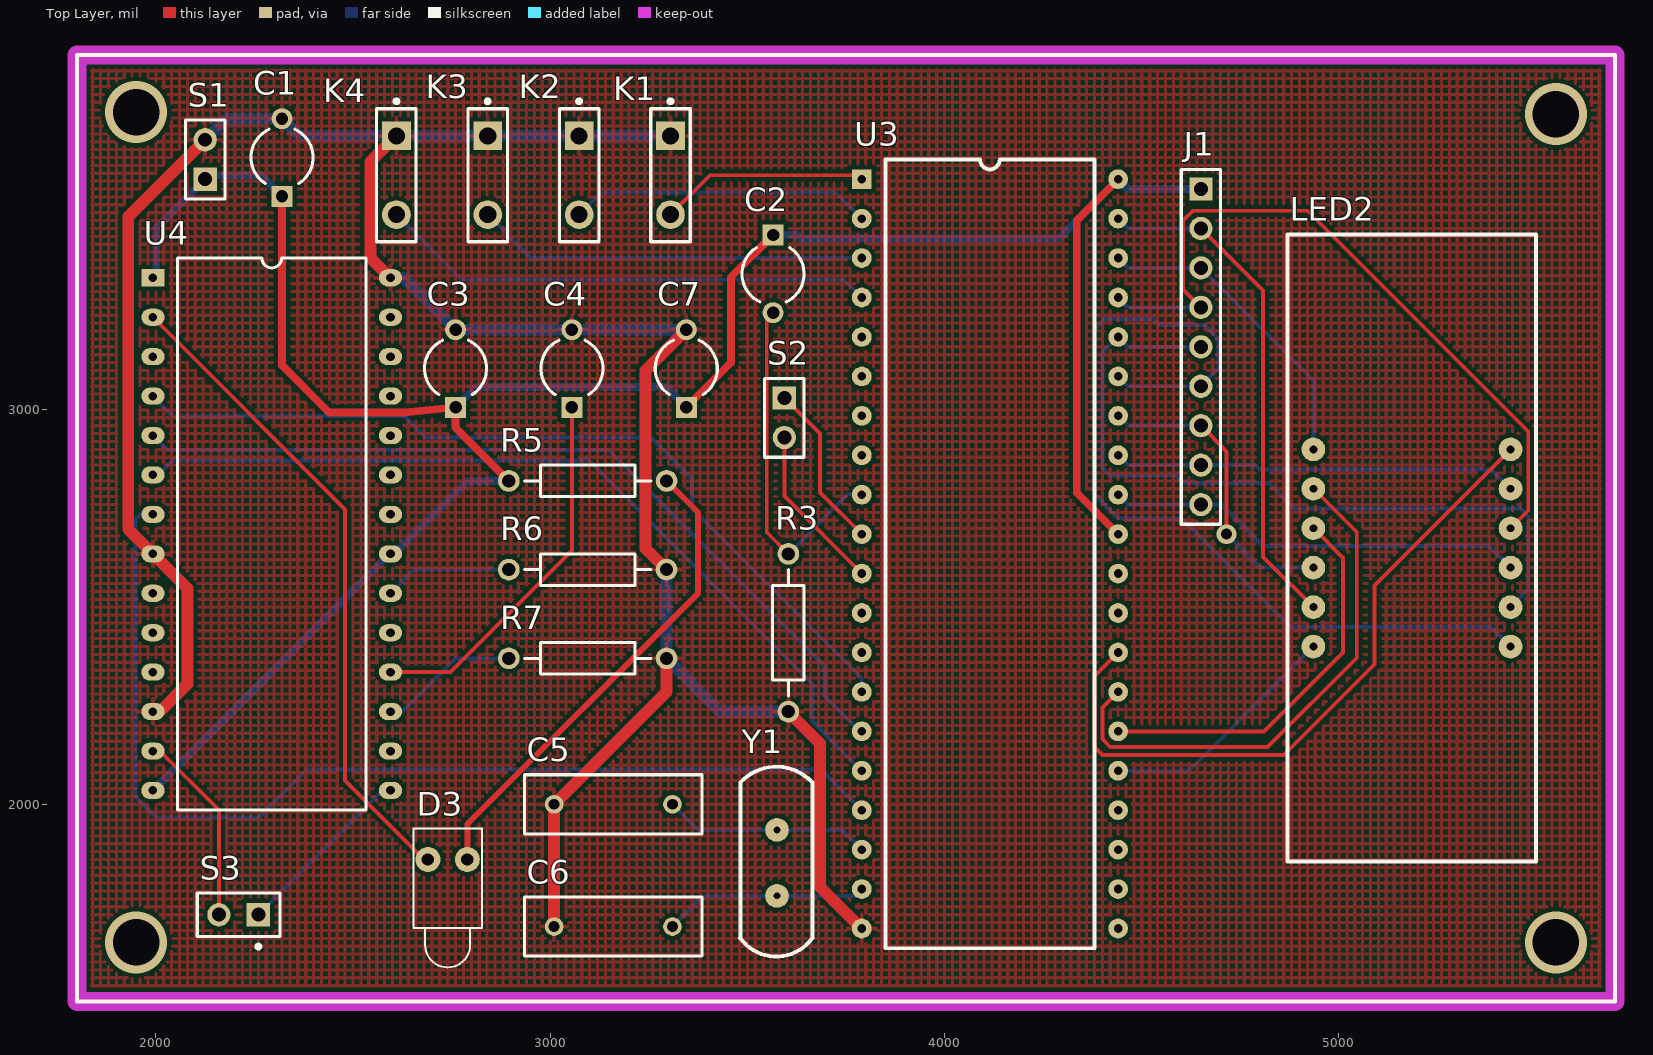
[diagram p0: Top Layer view]
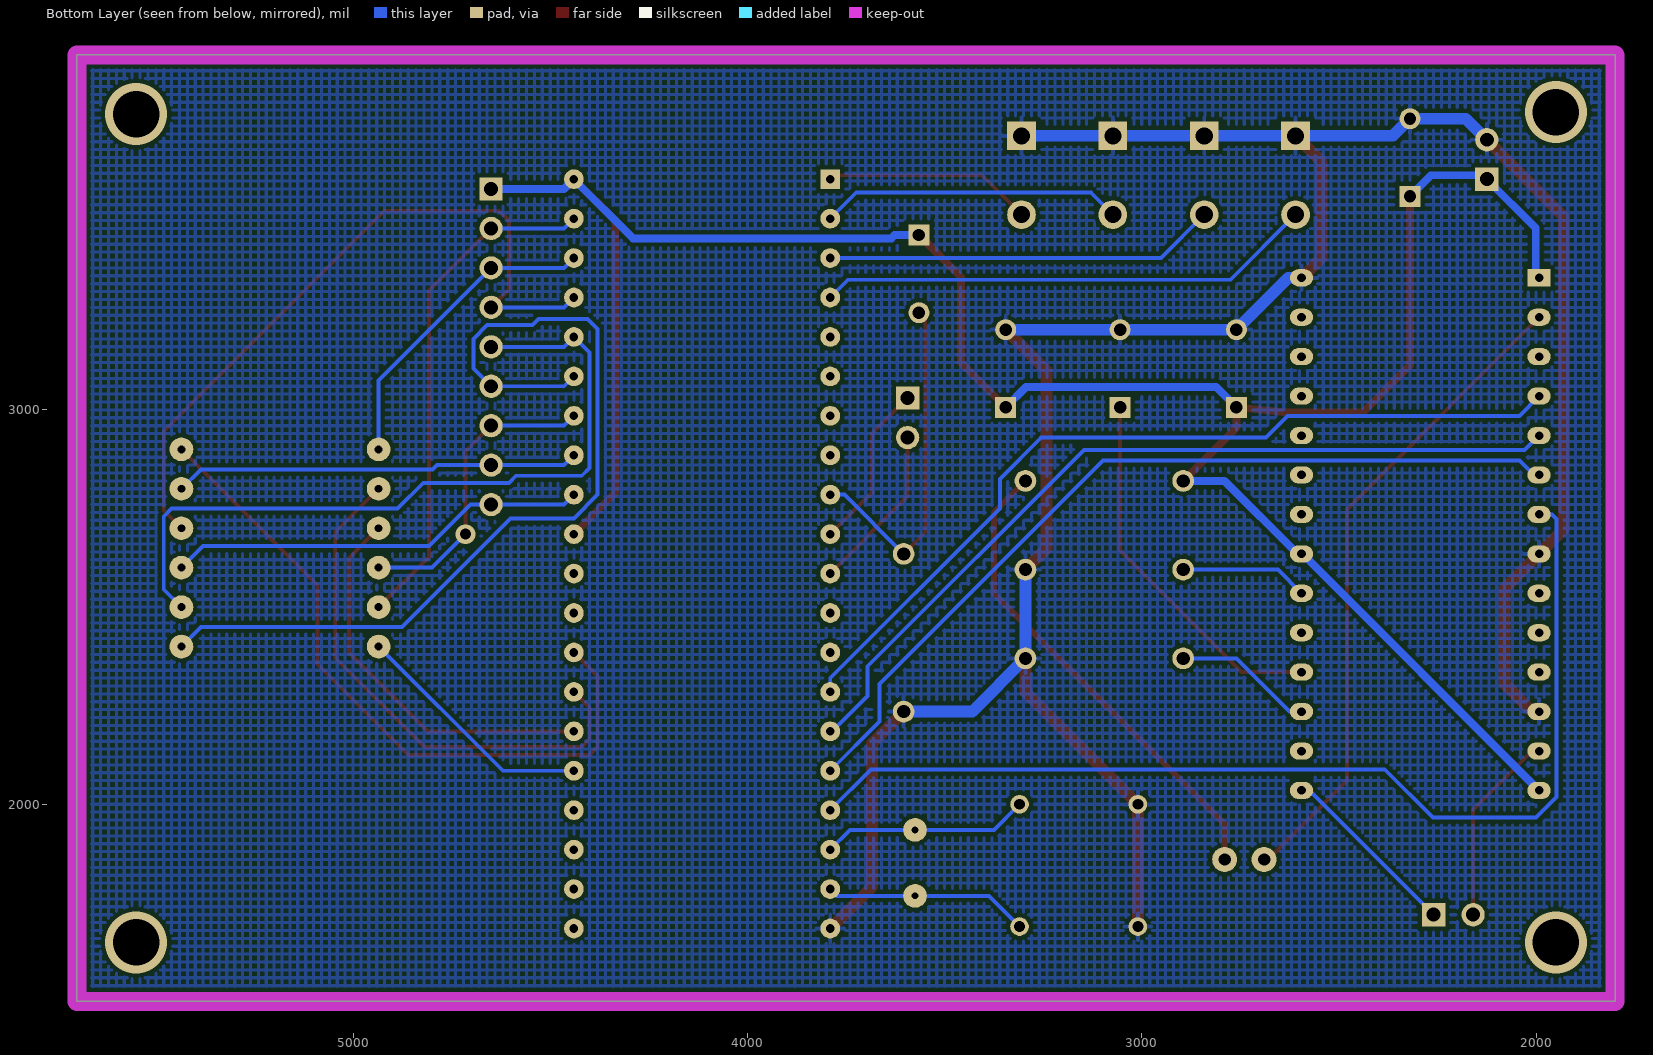
[diagram p1: Bottom Layer view, seen from below]
# Altium PCB MISC86338.PcbDoc
Units mil, origin at the board's own origin, x right, y up, seen from the top; angles counter-clockwise.
Board outline 3900 x 2400 mil, 2 copper layers (Top Layer, Bottom Layer); 24 components, 34 nets, 129 pads, 5 vias.

## Layer stack, top to bottom (the 12.6 mil dielectric is the usual default, probably not edited)
Top Solder: solder mask 0.4, Solder Resist, Dk 3.5
Top Layer: signal copper 1.4
Dielectric 1: dielectric 12.6, FR-4, Dk 4.8
Bottom Layer: signal copper 1.4
Bottom Solder: solder mask 0.4, Solder Resist, Dk 3.5

## Board outline
1800,1500 5700,1500 5700,3900 1800,3900

## Design rules (kind name [scope] priority, off if disabled: settings)
Clearance [All] p1: gap=10
HoleSize [All] p1: absolutevalues=TRUE maxlimit=500 minlimit=1 maxpercent=80.000 minpercent=20.000
MinimumSolderMaskSliver [All] p1: minsoldermaskwidth=5
PolygonConnect [All] p1: connectstyle=Relief reliefconductorwidth=10 reliefentries=4 polygonreliefangle="90 Angle" airgapwidth=10
RoomDefinition 公交自动报站器 [InComponentClass('公交自动报站器')] p1: confinementstyle=ConfineIn formatcopy=TRUE lockcomponents=FALSE outline 1800,1500 5700,1500 5700,3900 1800,3900
RoutingVias [All] p1: holewidth=28 width=50 viastyle="Through Hole" minholewidth=28 minwidth=50 maxholewidth=28 maxwidth=50
SilkToSolderMaskClearance [IsPad] p1: minsilkscreentomaskgap=0 clearancetoexposedcopper=TRUE
SolderMaskExpansion [All] p1: expansion=4
Width GND [InNet('GND')] p1: maxlimit=35 minlimit=10 preferedwidth=30
Width VCC [InNet('VCC')] p2: maxlimit=25 minlimit=10 preferedwidth=20
Width [All] p3: maxlimit=15 minlimit=8 preferedwidth=10
27 further rules are at their usual default settings.

## Components (designator, comment, footprint, x,y, rotation, side; value= is the part's Value field where it differs from the comment)
C1 "Cap2" CAPR5-4X5 2320,3640 r90 top
C2 "Cap2" CAPR5-4X5 3565,3345 r270 top
C3 "Cap2" CAPR5-4X5 2760,3105 r90 top
C4 "Cap2" CAPR5-4X5 3055,3105 r90 top
C5 "Cap" RAD-0.3 3160,2000 r0 top
C6 "Cap" RAD-0.3 3160,1690 r0 top
C7 "Cap2" CAPR5-4X5 3345,3105 r90 top
D3 "LED1" LED-1 2740,1860 r270 top
J1 "Header 9" HDR1X9 4650,3560 r270 top
K1 "SW-PB" SPST-2 3305,3595 r270 top
K2 "SW-PB" SPST-2 3073.33,3595 r270 top
K3 "SW-PB" SPST-2 2841.67,3595 r270 top
K4 "SW-PB" SPST-2 2610,3595 r270 top
LED2 "Dpy Red-CA" 四位数码管 5499.96,1854.72 r90 top
R3 "Res2" AXIAL-0.4 3603.74,2435 r90 top
R5 "Res2" AXIAL-0.4 3095,2820 r0 top
R6 "Res2" AXIAL-0.4 3095,2595 r180 top
R7 "Res2" AXIAL-0.4 3095,2370 r180 top
S1 "Header 2" HDR1X2 2125,3585 r90 top
S2 "Header 2" HDR1X2 3593.74,3030 r270 top
S3 "Speaker" PIN2 2260,1720 r180 top
U3 "89c51" 89c51 3790,3585 r0 top
U4 "Component_1" ISD1730 1992.64,3335 r0 top
Y1 "Component_1" XTAL 3665,2055 r180 top

## Footprints (in the part's own frame and the unit in brackets; to place one, negate y for a bottom-side part, rotate by r counter-clockwise, add the part's x,y. Pads: shape width x height; smd on the part's side, far side on the other; paste and mask are expansions set on the pad)
89c51 [mil]
  rect 50x50 hole 22: 1(0,0)
  round 50 hole 22: 2(0,-100) 3(0,-200) 4(0,-300) 5(0,-400) 6(0,-500) 7(0,-600) 8(0,-700) 9(0,-800) 10(0,-900) 11(0,-1000) 12(0,-1100) 13(0,-1200) 14(0,-1300) 15(0,-1400) 16(0,-1500) 17(0,-1600) 18(0,-1700) 19(0,-1800) 20(0,-1900) 21(650,-1900) 22(650,-1800) 23(650,-1700) 24(650,-1600) 25(650,-1500) 26(650,-1400) 27(650,-1300) 28(650,-1200) 29(650,-1100) 30(650,-1000) 31(650,-900) 32(650,-800) 33(650,-700) 34(650,-600) 35(650,-500) 36(650,-400) 37(650,-300) 38(650,-200) 39(650,-100) 40(650,0)
  silkscreen extent 60,-1950 590,50, body extent 65,-1950 590,55, height 190
AXIAL-0.4 [mm] "Axial Device, Thru-Hole; 2 Leads; 0.4 in Pin Spacing"
  round 1.4 hole 0.85: 1(-5.08,0) 2(5.08,0)
  silkscreen extent -4.06,-1.02 4.06,1.02
CAPR5-4X5 [mm] "Capacitor; 2 Leads"
  rect 1.35x1.35 hole 0.8: 1(-2.5,0)
  round 1.35 hole 0.8: 2(2.5,0)
  silkscreen extent -1.69,-2 1.82,2
HDR1X2 [mm] "Connector; Header; 2 Position"
  rect 1.5x1.5 hole 0.9: 1(0,0)
  round 1.5 hole 0.9: 2(2.54,0)
  silkscreen extent -1.27,-1.27 3.81,1.27
HDR1X9 [mm] "Connector; Header; 9 Position"
  rect 1.5x1.5 hole 0.9: 1(0,0)
  round 1.5 hole 0.9: 2(2.54,0) 3(5.08,0) 4(7.62,0) 5(10.16,0) 6(12.7,0) 7(15.24,0) 8(17.78,0) 9(20.32,0)
  silkscreen extent -1.27,-1.27 21.59,1.27
ISD1730 [mm]
  rect 1.5x1.1 hole 0.55: 1(0,0)
  oval 1.5x1.1 hole 0.55: 2(0,-2.54) 3(0,-5.08) 4(0,-7.62) 5(0,-10.16) 6(0,-12.7) 7(0,-15.24) 8(0,-17.78) 9(0,-20.32) 10(0,-22.86) 11(0,-25.4) 12(0,-27.94) 13(0,-30.48) 14(0,-33.02) 15(15.3,-33.02) 16(15.3,-30.48) 17(15.3,-27.94) 18(15.3,-25.4) 19(15.3,-22.86) 20(15.3,-20.32) 21(15.3,-17.78) 22(15.3,-15.24) 23(15.3,-12.7) 24(15.3,-10.16) 25(15.3,-7.62) 26(15.3,-5.08) 27(15.3,-2.54) 28(15.3,0)
  silkscreen extent 1.59,-34.29 13.71,1.27
LED-1 [mm] "LED; 2 Leads"
  round 1.6 hole 0.8: 1(0,1.27) 2(0,-1.27)
  silkscreen extent -2,-2.2 6.95,2.2
PIN2 [mm] "Photosensitive Diode; 2 Leads"
  rect 1.5x1.5 hole 0.9: 1(0,0)
  round 1.5 hole 0.9: 2(2.54,0)
  silkscreen extent -1.4,-1.4 3.94,2.17
RAD-0.3 [mm] "Radial Cap, Thru-Hole; 2 Leads; 0.3 in Pin Spacing"
  round 1.2 hole 0.7: 1(-3.81,0) 2(3.81,0)
  silkscreen extent -5.71,-1.91 5.71,1.91
SPST-2 [mm] "Switch; 2 Leads"
  rect 1.85x1.85 hole 1.1: 1(-2.54,0)
  round 1.85 hole 1.1: 2(2.54,0)
  silkscreen extent -4.89,-1.27 4.28,1.27
XTAL [mil]
  round 60 hole 17.13: 1(90,287.13) 2(90,120)
  silkscreen extent 0,-40 184,441
四位数码管 [mm]
  round 1.524 hole 0.51: 1(13.85,1.65) 2(16.39,1.65) 3(18.93,1.65) 4(21.47,1.65) 5(24.01,1.65) 6(26.55,1.65) 7(26.55,14.35) 8(24.01,14.35) 9(21.47,14.35) 10(18.93,14.35) 11(16.39,14.35) 12(13.85,14.35)
  silkscreen extent 0,0 40.4,16

## Part data
C1 C2 C3 C4 C5 C6 C7: "Capacitor"
D3: "Typical RED GaAs LED"
J1: "Header, 9-Pin"
K1 K2 K3 K4: "Switch"
LED2: "7.62 mm Black Surface HER 7-Segment Display: CA, RH DP"
R3 R5 R6 R7: "Resistor"
S1 S2: "Header, 2-Pin"
S3: "Loudspeaker"
U3: library part Component_1

## Via types
v1: diameter 157.48, hole 118.11, Top Layer to Bottom Layer, 4 vias
v2: diameter 50, hole 28, Top Layer to Bottom Layer, 1 vias

## Nets (pads, with @x,y where several pads share a name; then routed paths per layer and width w, separated by ;. In a path a pad name is that pad's centre, name@x,y a point inside that pad or via, vN(x,y) a via of type N, cw(c..) or ccw(c..) an arc to the next point about the centre after c; other vN are vias at no path point)
GND: C1.2 C3.2 C4.2 C5.1 C6.1 C7.2 K1.1 K2.1 K3.1 K4.1 R3.1 R6.1 R7.1 S1.2 U3.20 U4.8 U4.12 U4.28 | length 6760.2
  Top Layer w30: U4.12 2010,2235 2080,2305 2080,2547.64 U4.8 1930,2697.64 1930,3490 S1.2 ; U4.28 2544,3386 2544,3629 K4.1 ; C6.1 C5.1 3295,2285 R7.1 ; R6.1 3242,2648 3242,3100.43 C7.2 ; R3.1 3684,2154.74 3684,1791 U3.20
  Bottom Layer w30: S1.2 2178.43,3738.43 C1.2 2363.43,3695 K4.1 K3.1 K2.1 K1.1 ; U4.28 2628.43,3335 C3.2 C4.2 C7.2 ; R6.1 R7.1 3430,2235 R3.1
NetC2_2: C2.2 R3.2 U3.9 | length 898.6
  Top Layer w10: C2.2 3565,3228 3549,3228 3549,2689.74 R3.2
  Bottom Layer w10: R3.2 3753.74,2785 U3.9
NetC4_1: C4.1 U4.18 | length 951.2
  Top Layer w10: U4.18 2747,2335 3055,2643 C4.1
NetC5_2: C5.2 U3.18 Y1.2 | length 527.6
  Bottom Layer w10: C5.2 3375,1935 Y1.2 3740,1935 U3.18
NetC6_2: C6.2 U3.19 Y1.1 | length 519.4
  Bottom Layer w10: C6.2 3387.87,1767.87 Y1.1 3772.87,1767.87 U3.19
NetD3_1: D3.1 R5.2 | length 1235.5
  Top Layer w15: D3.1 2790,1950 3375,2535 3375,2740 R5.2
NetD3_2: D3.2 U4.2 | length 1669.7
  Top Layer w10: U4.2 2480,2747.64 2480,2060 2680,1860 D3.2
NetR6_2: R6.2 U4.20 | length 324.9
  Bottom Layer w10: U4.20 2655,2595 R6.2
NetR7_2: R7.2 U4.17 | length 355.9
  Bottom Layer w10: U4.17 2625,2235 2760,2370 R7.2
NetS2_1: S2.1 U3.10 | length 426.3
  Top Layer w10: S2.1 3684,2939.74 3684,2791 U3.10
NetS2_2: S2.2 U3.11 | length 426.3
  Top Layer w10: S2.2 3593.74,2781.26 U3.11
NetS3_1: S3.1 U4.15 | length 465.5
  Bottom Layer w10: S3.1 2575,2035 U4.15
NetS3_2: S3.2 U4.13 | length 494.5
  Top Layer w10: U4.13 2010,2135 2160,1985 S3.2
P00: J1.2 LED2.11 U3.39 | length 1298.4
  Top Layer w10: J1.2 4807.47,3302.53 4807.47,2627.53 LED2.11
  Bottom Layer w10: U3.39 4465,3460 J1.2
P01: J1.3 LED2.7 U3.38 | length 798.4
  Bottom Layer w10: U3.38 4465,3360 J1.3 4935,3075 LED2.7
P02: J1.4 LED2.4 U3.37 | length 1839.9
  Top Layer w10: J1.4 4605,3305 4605,3480 4630,3505 4920,3505 5480,2945 5480,2745 LED2.4
  Bottom Layer w10: U3.37 4465,3260 J1.4
P03: J1.5 LED2.2 U3.36 | length 1948.5
  Bottom Layer w10: J1.5 4465,3160 U3.36 4400,3145 4400,2853 4420,2833 4587,2833 4605,2815 4822,2815 4887,2750 5460,2750 5480,2730 5480,2545 LED2.2
P04: J1.6 LED2.1 U3.35 | length 2339.5
  Bottom Layer w10: U3.35 4465,3060 J1.6 4695,3105 4695,3180 4660,3215 4545,3215 4530,3230 4405,3230 4380,3205 4380,2785 4440,2725 4601,2725 4876,2450 5385,2450 LED2.1
P05: J1.7 LED2.10 U3.34 | length 777.5
  Top Layer w10: J1.7 4715,2895 v2(4715,2685)
  Bottom Layer w10: U3.34 4465,2960 J1.7 ; v2(4715,2685) 4800,2600 LED2.10
P06: J1.8 LED2.5 U3.33 | length 1030.2
  Bottom Layer w10: U3.33 4465,2860 J1.8 4787,2860 4798,2849 5386,2849 LED2.5
P07: J1.9 LED2.3 U3.32 | length 1071.6
  Bottom Layer w10: U3.32 4465,2760 J1.9 4702.47,2760 4807.47,2655 5380,2655 LED2.3
P10: K1.2 U3.1 | length 530.6
  Top Layer w10: K1.2 3405,3595 3780,3595 U3.1
P11: K2.2 U3.2 | length 767.2
  Bottom Layer w10: K2.2 3129.33,3551 3724,3551 U3.2
P12: K3.2 U3.3 | length 993.9
  Bottom Layer w10: K3.2 2951.67,3385 U3.3
P13: K4.2 U3.4 | length 1267
  Bottom Layer w10: K4.2 2775,3330 3745,3330 U3.4
P24: LED2.12 U3.25 | length 625.5
  Bottom Layer w10: U3.25 4620,2085 LED2.12
P25: LED2.9 U3.26 | length 998.9
  Top Layer w10: U3.26 4810,2185 5010,2385 5010,2625 LED2.9
P26: LED2.8 U3.27 | length 1358
  Top Layer w10: U3.27 4400,2245 4400,2165 4420,2145 4819,2145 5045,2371 5045,2690 LED2.8
P27: LED2.6 U3.28 | length 1766.3
  Top Layer w10: U3.28 4380,2325 4380,2145 4400,2125 4860,2125 5090,2355 5090,2555 LED2.6
P34: U3.14 U4.4 | length 2172.5
  Bottom Layer w10: U4.4 2042.64,2985 2630,2985 2685,2930 3255,2930 3360,2825 3360,2750 3790,2320 U3.14
P35: U3.15 U4.5 | length 2152
  Bottom Layer w10: U4.5 2029.29,2898.35 3146.65,2898.35 3695,2350 3695,2275 3785,2185 U3.15
P36: U3.16 U4.6 | length 2194.3
  Bottom Layer w10: U4.6 2005,2835 2042,2872 3098,2872 3665,2305 3665,2210 U3.16
P37: U3.17 U4.7 | length 2711.3
  Bottom Layer w10: U4.7 1960,2735 1948,2723 1948,2018 2000,1966 2262,1966 2384,2088 3687,2088 U3.17
VCC: C1.1 C2.1 C3.1 C7.1 J1.1 R5.1 S1.1 U3.31 U3.40 U4.1 U4.14 U4.21 | length 6223.5
  Top Layer w20: C1.1 2320,3113 2440,2993 2631.43,2993 C3.1 2760,2955 R5.1 ; C7.1 3458,3119.57 3458,3336.43 C2.1 ; U3.31 4335,2790 4335,3480 U3.40
  Bottom Layer w20: U4.14 2592.64,2635 U4.21 2605,2635 2790,2820 R5.1 ; U4.1 2001,3335 2001,3461 S1.1 2135,3595 2266.57,3595 C1.1 ; C3.1 2811.43,3058 3293.57,3058 C7.1 ; C2.1 3626.57,3443.43 3635,3435 4290,3435 U3.40 4465,3560 J1.1
pads on no net: U3.5 U3.6 U3.7 U3.8 U3.12 U3.13 U3.21 U3.22 U3.23 U3.24 U3.29 U3.30 U4.3 U4.9 U4.10 U4.11 U4.16 U4.19 U4.22 U4.23 U4.24 U4.25 U4.26 U4.27
copper on no net:
  other v1: 1950,1650 5550,1650 5550,3750 1950,3755

## Polygon pours and split planes (outlines as drawn)
GND on Top Layer "Top Layer-No Net" (hatched 90Degree grid 20 track 8, pour order 0): 1800,3900 1810,3890 5700,3890 5700,1500 1800,1500
GND on Bottom Layer "Top Layer-No Net" (hatched 90Degree grid 20 track 8, pour order 2): 1800,3900 5700,3900 5700,1500 1810,1500 1800,1510

## Keep-outs
Keep-Out Layer:
  the board outline again, w47.24

## Silkscreen, mask and mechanical layers (free items; w line width, h text height)
Top Overlay:
  the board outline again, w10